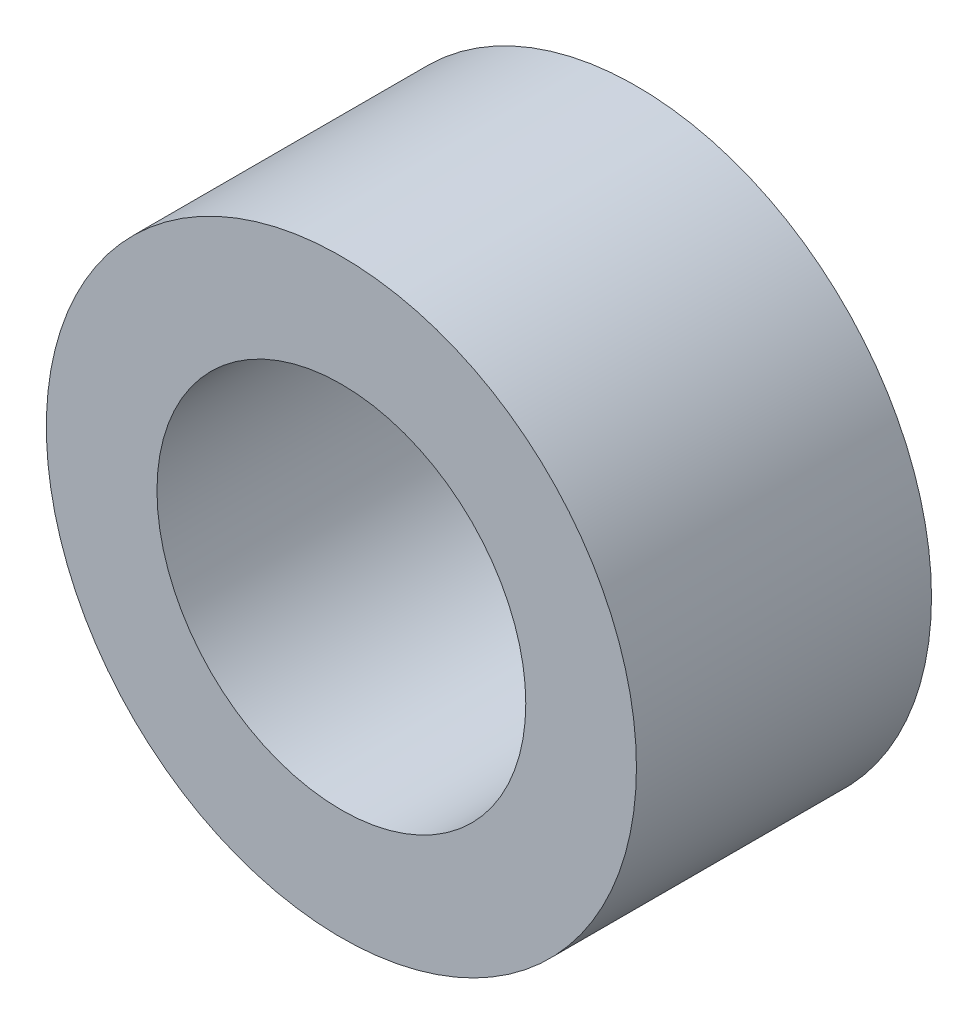
from build123d import *

# Parameters (mm, degrees)
SKETCH1_R           = 5
SKETCH1_R_2         = 3.125
BOSS_EXTRUDE1_DEPTH = 5


with BuildPart() as part:
    # Sketch1 → Boss-Extrude1 (new body)
    with BuildSketch(Plane.XY):
        Circle(SKETCH1_R)
        Circle(SKETCH1_R_2, mode=Mode.SUBTRACT)
    extrude(amount=BOSS_EXTRUDE1_DEPTH)


solid = part.part
